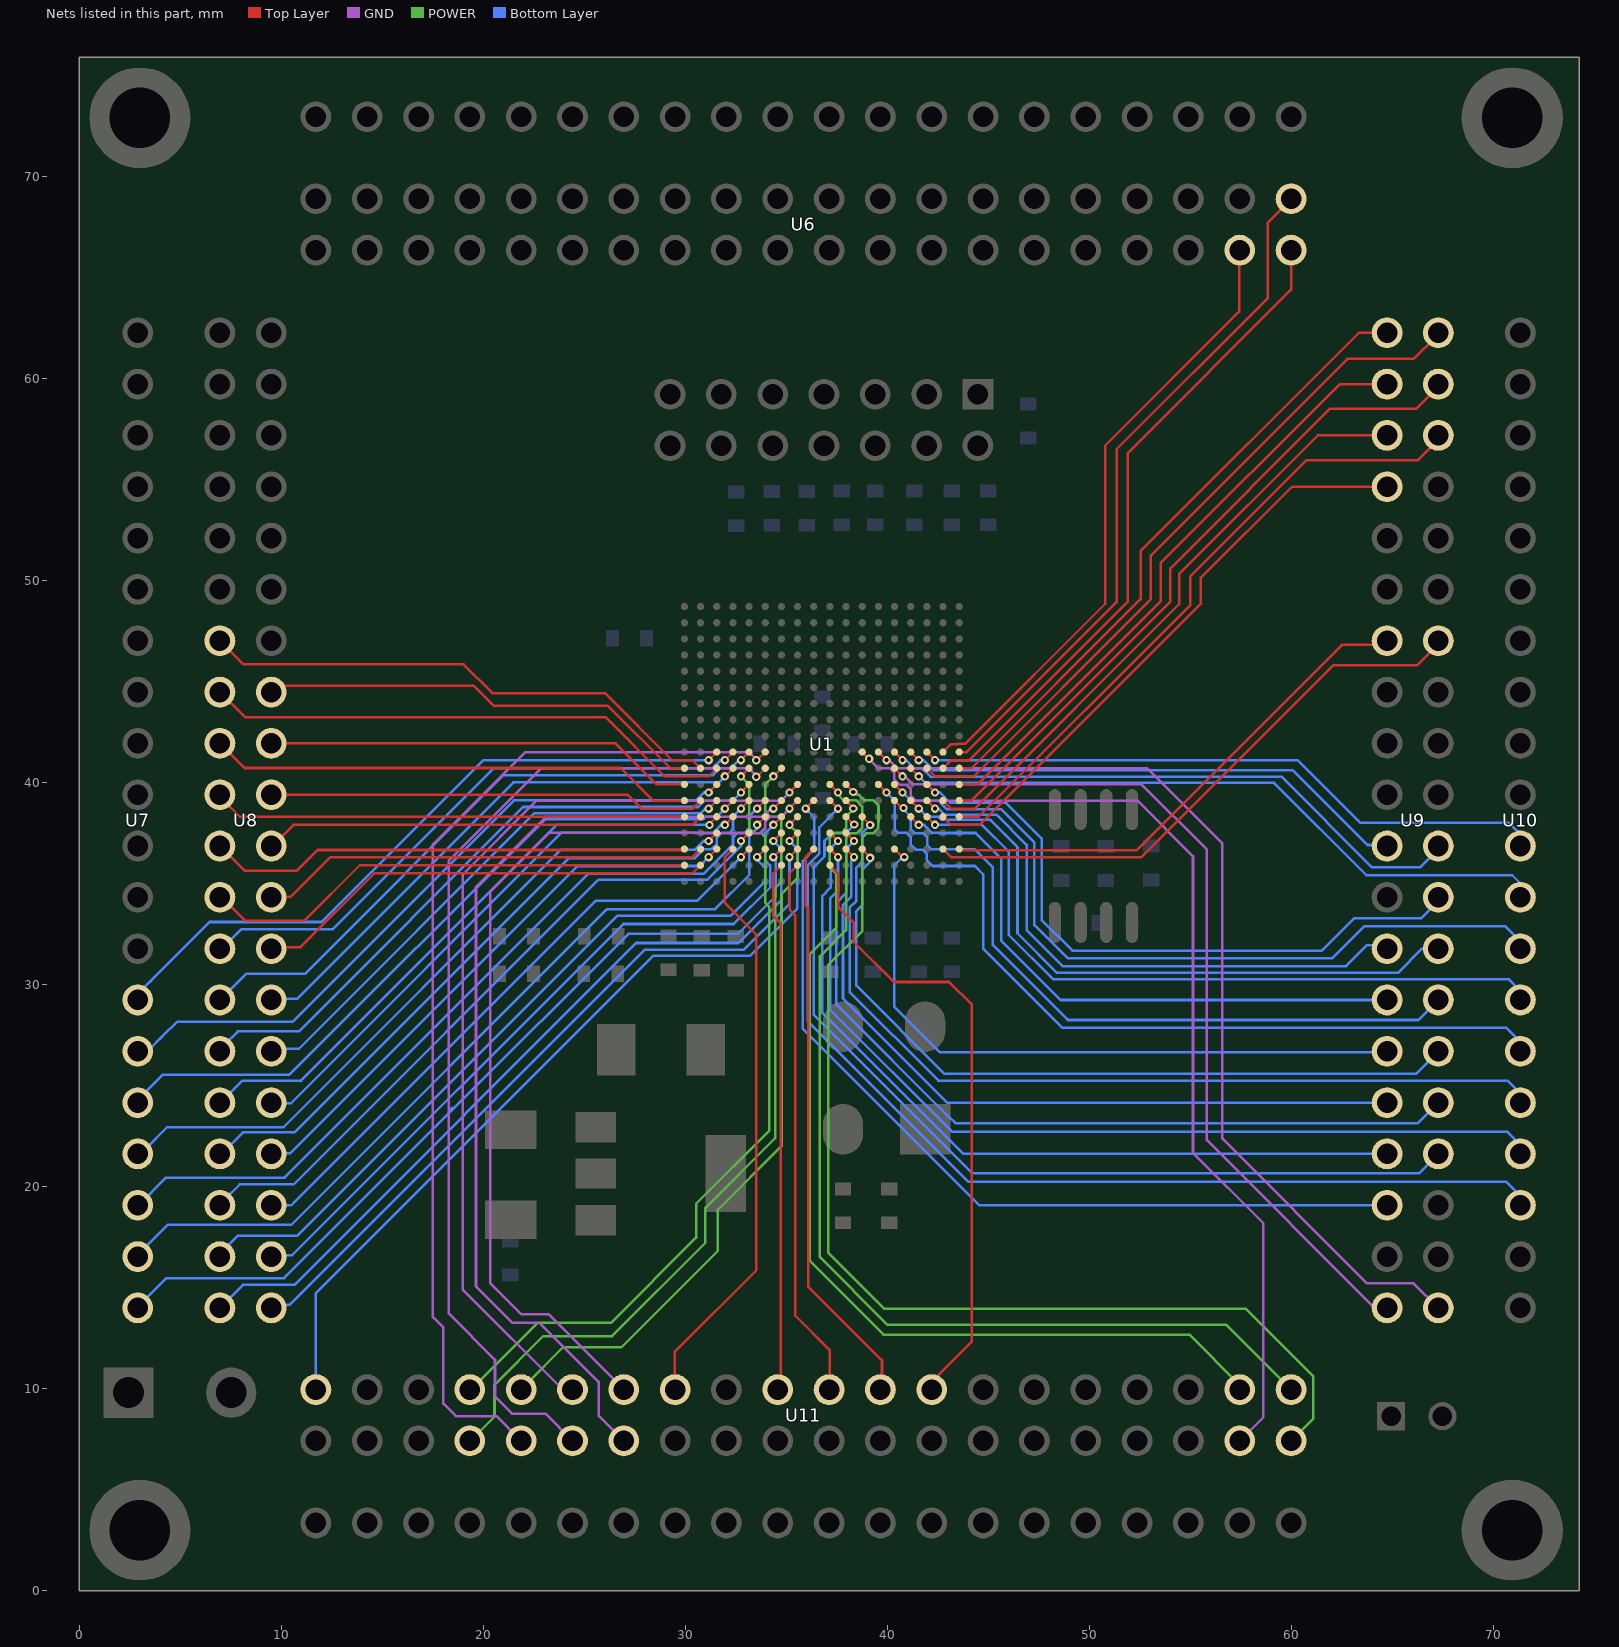
[diagram p0: the nets of this part, all layers, seen from the top]
# Altium PCB MISC103828.PcbDoc (part 3 of 4)
Units mm, origin at the board's own origin, x right, y up, seen from the top; angles counter-clockwise.
Board outline 74.24 x 75.89 mm, 4 copper layers (Top Layer, GND, POWER, Bottom Layer); 49 components, 246 nets, 670 pads, 283 vias.

## Via types
v1: diameter 0.406, hole 0.203, Top Layer to Bottom Layer, 221 vias
v2: diameter 0.61, hole 0.305, Top Layer to Bottom Layer, 43 vias
v3: diameter 0.508, hole 0.254, Top Layer to Bottom Layer, 16 vias
v4: diameter 0.432, hole 0.229, Top Layer to Bottom Layer, 3 vias

## Nets (pads, with @x,y where several pads share a name; then routed paths per layer and width w, separated by ;. In a path a pad name is that pad's centre, name@x,y a point inside that pad or via, vN(x,y) a via of type N, cw(c..) or ccw(c..) an arc to the next point about the centre after c; other vN are vias at no path point) (continued)
F_K3: U1.K3 U7.14 | length 34.1
  Top Layer w0.127: v1(31.147,41.103) U1.K3@31.547,41.503
  Bottom Layer w0.127: U7.14@2.845,29.286 2.845,29.489 3.556,30.201 ; 3.505,30.15 3.556,30.201 ; 22.993,41.103 23.139,41.103 ; v1(31.147,41.103) 23.139,41.103 ; 3.556,30.201 6.452,33.096 11.989,33.096 19.996,41.103 23.139,41.103
F_K4: U1.K4 U8.25 | length 29.1
  Top Layer w0.127: v1(31.947,41.103) U1.K4@32.347,41.503
  Bottom Layer w0.127: U8.25@7.239,31.953 8.014,32.728 12.535,32.728 20.517,40.71 31.337,40.71 31.725,41.097 v1@31.928,41.097 ; v1@31.935,41.09 v1(31.947,41.103)
F_K5: U1.K5 U8.27 | length 30.8
  Top Layer w0.127: v1(32.747,41.103) U1.K5@33.147,41.503
  Bottom Layer w0.127: U8.27@7.29,29.566 8.255,30.531 11.176,30.531 21.006,40.361 31.369,40.361 31.718,40.71 32.251,40.71 32.645,41.103 v1(32.747,41.103)
F_K6: U1.K6 U11.9 | length 51.3
  Top Layer w0.127: v1(33.503,41.097) 33.503,41.123 33.528,41.123 33.547,41.103 U1.K6@33.947,41.503
  GND w0.127: U11.9@21.869,7.417 20.65,8.636 18.644,8.636 18.021,9.258 18.021,13.018 17.501,13.538 17.501,36.932 22.073,41.504 33.147,41.504 33.528,41.123 33.503,41.123 v1(33.503,41.097)
F_K12: U1.K12 U11.37 | length 49.8
  Top Layer w0.127: U1.K12@38.747,41.503 39.091,41.16 v1(39.091,41.173)
  GND w0.127: v1(39.091,41.173) 39.091,41.16 39.554,40.697 40.11,40.697 40.341,40.466 40.341,40.153 40.597,39.897 40.91,39.897 41.141,39.666 41.141,39.353 41.397,39.097 52.368,39.097 55.118,36.347 55.118,21.666 58.598,18.186 58.598,8.585 U11.37@57.429,7.417
F_K13: U1.K13 U9.40 | length 47.7
  Top Layer w0.127: U1.K13@39.547,41.503 v1(39.947,41.103)
  GND w0.127: v1(39.947,41.103) 40.063,41.103 40.457,40.71 52.839,40.71 56.566,36.982 56.566,22.377 63.729,15.215 66.04,15.215 U9.40@67.259,13.995
F_K14: U1.K14 U9.22 | length 29.7
  Top Layer w0.127: U1.K14@40.347,41.503 v1(40.747,41.103)
  Bottom Layer w0.127: v1(40.747,41.103) 40.913,41.103 41.32,40.697 41.71,40.697 42.123,40.284 59.487,40.284 63.957,35.814 66.37,35.814 U9.22@67.335,36.779
F_K15: U1.K15 U9.21 | length 25.3
  Top Layer w0.127: U1.K15@41.147,41.503 v1(41.547,41.103)
  Bottom Layer w0.127: v1(41.547,41.103) 41.777,41.103 42.266,40.615 60.046,40.615 63.754,36.906 U9.21@64.567,36.906
F_K16: U1.K16 U10.11 | length 31.8
  Top Layer w0.127: U1.K16@41.947,41.503 v1(42.347,41.103)
  Bottom Layer w0.127: v1(42.347,41.103) 60.293,41.103 63.398,37.998 70.764,37.998 U10.11@71.857,36.906
F_K17: U1.K17 U6.37 | length 31.1
  Top Layer w0.127: U1.K17@42.747,41.503 43.143,41.899 43.485,41.899 43.485,41.907 43.838,41.907 50.775,48.844 50.775,56.667 57.404,63.297 57.404,66.015 U6.37@57.353,66.065
F_K18: U1.K18 U6.40 | length 34.5
  Top Layer w0.127: U1.K18@43.547,41.503 43.916,41.503 51.333,48.92 51.333,56.49 58.826,63.983 58.826,67.71 59.249,68.132 ; 59.293,68.177 59.249,68.132 ; U6.40@59.969,68.936 59.969,68.853 59.249,68.132
F_L1: U1.L1 U8.16 | length 22.3
  Top Layer w0.127: U8.16@9.5,44.475 9.804,44.78 19.533,44.78 19.837,44.475 19.875,44.437 20.523,43.79 26.162,43.79 29.248,40.703 U1.L1@29.947,40.703
F_L2: U1.L2 U8.13 | length 26.4
  Top Layer w0.127: U8.13@6.96,47.015 8.128,45.847 19.025,45.847 20.447,44.425 26.01,44.425 29.335,41.099 30.352,41.099 U1.L2@30.747,40.703
F_L3: U1.L3 U8.15 | length 26.5
  Top Layer w0.127: U8.15@6.96,44.475 8.204,43.231 26.035,43.231 28.958,40.307 30.111,40.307 30.114,40.31 30.581,40.31 30.583,40.307 31.152,40.307 U1.L3@31.547,40.703
F_L4: U1.L4 U8.28 | length 27.4
  Top Layer w0.127: v1(31.947,40.303) U1.L4@32.347,40.703
  Bottom Layer w0.127: U8.28@9.677,29.286 10.77,29.286 21.488,40.005 31.649,40.005 v1(31.947,40.303)
F_L5: U1.L5 U11.8 | length 39.6
  Top Layer w0.127: v1(32.747,40.303) U1.L5@33.147,40.703
  POWER w0.127: U11.8@19.66,10.236 22.682,13.259 26.314,13.259 30.531,17.475 30.531,19.152 34.138,22.758 34.138,33.858 33.954,34.042 33.954,37.266 33.967,37.28 33.75,37.497 33.397,37.497 33.154,37.74 33.154,39.897 v1(32.747,40.303)
F_L6: U1.L6 U11.11 | length 50.3
  Top Layer w0.127: v1(33.503,40.284) 33.494,40.284 33.494,40.252 33.496,40.252 U1.L6@33.947,40.703
  GND w0.127: U11.11@24.409,7.417 23.063,8.763 21.412,8.763 20.574,9.601 20.574,11.43 18.288,13.716 18.288,36.144 22.841,40.697 33.154,40.697 33.547,40.303 33.496,40.252 33.494,40.252 33.494,40.284 v1(33.503,40.284)
F_L7: U1.L7 U11.7 | length 42.7
  Top Layer w0.127: v1(34.347,40.303) U1.L7@34.747,40.703
  POWER w0.127: U11.7@19.228,7.29 20.549,8.611 20.549,10.185 22.962,12.598 26.365,12.598 30.988,17.221 30.988,18.948 34.442,22.403 34.442,34.239 34.442,34.315 34.442,34.773 34.747,35.077 34.747,38.125 34.563,38.31 34.184,38.31 33.941,38.553 33.941,38.583 33.941,39.897 v1(34.347,40.303)
F_L14: U1.L14 U9.39 | length 43.9
  Top Layer w0.127: U1.L14@40.347,40.703 v1(40.747,40.303)
  GND w0.127: v1(40.747,40.303) 40.863,40.303 41.263,39.903 52.578,39.903 55.804,36.678 55.804,22.301 64.11,13.995 U9.39@64.719,13.995
F_L15: U1.L15 U10.12 | length 33.3
  Top Layer w0.127: U1.L15@41.147,40.703 v1(41.547,40.303)
  Bottom Layer w0.127: v1(41.547,40.303) 41.871,39.98 59.131,39.98 63.703,35.408 70.917,35.408 U10.12@71.857,34.468
F_L16: U1.L16 U9.2 | length 35.7
  Top Layer w0.127: U1.L16@41.947,40.703 42.343,40.307 44.27,40.307 53.035,49.073 53.035,51.232 62.763,60.96 64.465,60.96 66.04,60.96 U9.2@67.208,62.128
F_L17: U1.L17 U6.39 | length 33.2
  Top Layer w0.127: U1.L17@42.747,40.703 43.129,41.085 43.37,41.085 43.383,41.099 43.711,41.099 43.725,41.085 44.032,41.085 51.892,48.946 51.892,56.312 59.969,64.389 59.969,66.142 U6.39@60.046,66.218
F_L18: U1.L18 U9.1 | length 31.5
  Top Layer w0.127: U1.L18@43.547,40.703 44.158,40.703 52.527,49.073 52.527,51.46 63.322,62.255 U9.1@64.719,62.255
F_M1: U1.M1 U8.18 | length 21.3
  Top Layer w0.127: U8.18@9.5,41.935 26.543,41.935 28.575,39.903 U1.M1@29.947,39.903
F_M3: U1.M3 U7.15 | length 34.1
  Top Layer w0.127: v1(31.147,39.503) U1.M3@31.547,39.903
  Bottom Layer w0.127: U7.15@3.099,26.822 3.505,26.822 4.102,27.419 ; 3.988,27.305 4.102,27.419 ; 24.098,39.11 24.155,39.11 ; v1(31.147,39.503) 30.918,39.503 30.525,39.11 24.155,39.11 ; 4.102,27.419 4.851,28.169 10.566,28.169 21.508,39.11 24.155,39.11
F_M5: U1.M5 U8.29 | length 31.3
  Top Layer w0.127: v1(32.747,39.503) U1.M5@33.147,39.903
  Bottom Layer w0.127: U8.29@7.188,27.026 7.849,27.686 10.871,27.686 21.971,38.786 30.632,38.786 30.944,39.097 32.341,39.097 v1(32.747,39.503)
F_M8: U1.M8 U11.12 | length 46.4
  Top Layer w0.127: v1(35.147,39.503) U1.M8@35.547,39.903
  GND w0.127: U11.12@24.409,9.957 23.927,9.957 18.974,14.91 18.974,35.433 22.638,39.097 34.741,39.097 v1(35.147,39.503)
F_M10: U1.M10 U11.40 | length 51.4
  Top Layer w0.127: U1.M10@37.147,39.903 v1(37.547,39.503)
  POWER w0.127: v1@37.541,39.395 37.808,39.129 38.441,39.129 38.748,38.822 38.748,37.757 38.633,37.643 ; 38.638,37.638 38.498,37.497 38.184,37.497 37.954,37.266 37.954,32.696 36.652,31.394 36.652,16.51 40.005,13.157 56.769,13.157 U11.40@59.969,9.957
F_M11: U1.M11 U11.39 | length 55.7
  Top Layer w0.127: U1.M11@37.947,39.903 v1@38.341,39.51
  POWER w0.127: v1(38.303,39.522) 38.303,39.472 38.316,39.472 38.347,39.503 38.379,39.471 38.379,39.446 38.443,39.383 38.597,39.383 38.87,39.11 39.298,39.11 39.554,38.854 39.554,38.028 39.535,38.009 39.535,37.734 39.298,37.497 38.984,37.497 38.748,37.26 38.748,35.82 38.754,35.814 38.754,32.658 37.059,30.963 37.059,16.739 39.853,13.945 57.734,13.945 61.062,10.617 61.062,8.509 U11.39@59.969,7.417
F_M13: U1.M13 U10.15 | length 41.1
  Top Layer w0.127: U1.M13@39.547,39.903 v1(39.947,39.503)
  Bottom Layer w0.127: v1(39.947,39.503) 40.361,39.09 40.361,38.873 40.354,38.866 40.354,37.675 40.519,37.51 40.91,37.51 40.917,37.516 40.919,37.516 41.141,37.294 41.141,36.94 41.14,36.939 41.402,36.677 41.73,36.677 41.948,36.459 41.948,36.146 42.229,35.865 44.323,35.865 44.729,35.458 44.729,31.775 48.641,27.864 70.612,27.864 U10.15@71.78,26.695
F_M14: U1.M14 U10.13 | length 38.2
  Top Layer w0.127: U1.M14@40.347,39.903 v1(40.747,39.503)
  Bottom Layer w0.127: v1(40.747,39.503) 41.154,39.097 42.51,39.097 42.796,38.811 42.799,38.811 42.945,38.665 45.637,38.665 47.269,37.033 47.269,32.944 48.92,31.293 62.001,31.293 63.602,32.893 70.561,32.893 U10.13@71.501,31.953
F_M16: U1.M16 U9.24 | length 32
  Top Layer w0.127: U1.M16@41.947,39.903 v1(42.347,39.503)
  Bottom Layer w0.127: v1(42.347,39.503) 42.589,39.503 43.104,38.989 45.872,38.989 47.625,37.236 47.625,33.198 49.149,31.674 61.493,31.674 63.094,33.274 66.396,33.274 U9.24@67.208,34.087
F_M18: U1.M18 U9.3 | length 30.7
  Top Layer w0.127: U1.M18@43.547,39.903 44.45,39.903 53.53,48.984 ; 53.518,48.997 53.518,50.851 62.382,59.715 U9.3@64.719,59.715 ; U9.3@64.719,59.639 U9.3@64.922,59.639
F_N1: U1.N1 U8.17 | length 24.2
  Top Layer w0.127: U8.17@6.96,41.935 8.179,40.716 26.797,40.716 28.397,39.116 ; 28.397,39.103 U1.N1@29.947,39.103
F_N2: U1.N2 U8.20 | length 21.7
  Top Layer w0.127: U8.20@9.5,39.395 27.127,39.395 27.815,38.708 30.352,38.708 U1.N2@30.747,39.103
F_N3: U1.N3 U8.30 | length 27
  Top Layer w0.127: v1(31.147,38.703) U1.N3@31.547,39.103
  Bottom Layer w0.127: U8.30@9.601,26.822 10.871,26.822 22.53,38.481 30.759,38.481 30.982,38.703 v1(31.147,38.703)
F_N4: U1.N4 U7.16 | length 35.6
  Top Layer w0.127: v1(31.947,38.703) U1.N4@32.347,39.103
  Bottom Layer w0.127: U7.16@2.921,24.206 U7.16@3.277,24.206 ; U7.16@3.099,24.511 4.115,25.527 10.389,25.527 23.038,38.176 30.863,38.176 30.984,38.297 31.541,38.297 v1(31.947,38.703)
F_N5: U1.N5 U8.33 | length 33.5
  Top Layer w0.127: v1(32.747,38.703) U1.N5@33.147,39.103
  Bottom Layer w0.127: U8.33@7.341,21.92 8.103,22.682 10.643,22.682 24.206,36.246 30.455,36.246 30.906,36.697 31.298,36.697 31.554,36.953 31.554,37.269 31.795,37.51 32.176,37.51 32.36,37.694 32.36,37.734 32.354,37.74 32.354,38.066 32.36,38.072 32.36,38.316 v1(32.747,38.703)
F_N6: U1.N6 U7.18 | length 39.9
  Top Layer w0.127: v1(33.547,38.703) U1.N6@33.947,39.103
  Bottom Layer w0.127: U7.18@2.921,19.075 4.293,20.447 5.969,20.447 10.16,20.447 25.197,35.484 30.912,35.484 32.361,36.933 32.354,36.94 32.354,37.281 32.583,37.511 32.584,37.51 32.91,37.51 33.154,37.753 33.154,38.31 v1(33.547,38.703)
F_N7: U1.N7 U11.13 | length 48.1
  Top Layer w0.127: v1(34.347,38.703) U1.N7@34.747,39.103
  GND w0.127: U11.13@26.949,7.417 25.705,8.661 25.705,10.338 22.784,13.259 21.438,13.259 19.634,15.062 19.634,34.823 23.121,38.31 33.838,38.31 34.231,38.703 v1(34.347,38.703)
F_N8: U1.N8 U11.14 | length 45.4
  Top Layer w0.127: v1(35.147,38.703) U1.N8@35.547,39.103
  GND w0.127: U11.14@26.949,9.957 23.216,13.691 21.869,13.691 20.345,15.215 20.345,34.595 23.254,37.503 30.491,37.503 30.497,37.497 33.698,37.497 33.941,37.74 33.941,38.054 34.184,38.297 34.741,38.297 v1(35.147,38.703)
F_N9: U1.N9 U9.35 | length 44.4
  Top Layer w0.127: v1(35.947,38.703) U1.N9@36.347,39.103
  Bottom Layer w0.127: v1(35.947,38.703) 36.373,38.278 36.373,36.678 35.795,36.1 35.795,27.832 44.552,19.075 U9.35@64.719,19.075
F_N10: U1.N10 U10.18 | length 51.2
  Top Layer w0.127: U1.N10@37.147,39.103 v1(37.547,38.703)
  Bottom Layer w0.127: v1(37.547,38.703) 36.627,37.783 36.627,36.474 36.049,35.897 36.049,28.187 43.993,20.244 70.612,20.244 U10.18@71.78,19.075
F_N11: U1.N11 U11.38 | length 48.4
  Top Layer w0.127: U1.N11@37.947,39.103 v1@38.322,38.729 ; v1(38.303,38.71) v1@38.322,38.729 ; v1@38.322,38.729 38.329,38.735 38.329,38.722 v1@38.322,38.729
  POWER w0.127: 37.948,38.303 37.948,37.747 37.71,37.51 37.397,37.51 37.135,37.248 37.135,35.789 37.465,35.458 37.465,32.817 36.144,31.496 36.144,16.332 39.802,12.675 54.94,12.675 57.429,10.185 U11.38@57.429,9.957 ; 37.954,38.303 37.954,38.309 v1@38.354,38.71
F_N14: U1.N14 U9.28 | length 34.8
  Top Layer w0.127: U1.N14@40.347,39.103 40.747,38.703 40.767,38.723 40.767,38.735 v1(40.792,38.735)
  Bottom Layer w0.127: v1(40.792,38.735) 40.767,38.735 40.767,38.723 40.747,38.703 41.148,38.303 41.148,37.694 41.344,37.497 41.751,37.497 41.974,37.274 41.974,36.908 41.966,36.901 42.164,36.703 44.298,36.703 45.212,35.789 45.212,31.953 48.92,28.245 66.269,28.245 U9.28@67.259,29.235
F_N15: U1.N15 U9.26 | length 32.6
  Top Layer w0.127: U1.N15@41.147,39.103 v1(41.547,38.703)
  Bottom Layer w0.127: v1(41.547,38.703) 41.948,38.303 42.504,38.303 42.65,38.157 45.078,38.157 46.431,36.805 46.431,32.537 48.387,30.582 65.253,30.582 66.446,31.775 U9.26@67.259,31.775
F_N16: U1.N16 U9.25 | length 29.4
  Top Layer w0.127: U1.N16@41.947,39.103 v1(42.347,38.703)
  Bottom Layer w0.127: v1(42.347,38.703) 42.526,38.703 42.818,38.411 45.383,38.411 46.888,36.906 46.888,32.69 48.666,30.912 62.687,30.912 63.729,31.953 U9.25@65.024,31.953
F_N17: U1.N17 U9.5 | length 30.7
  Top Layer w0.127: U1.N17@42.747,39.103 43.143,38.708 44.321,38.708 54.432,48.819 54.432,50.317 61.29,57.175 U9.5@64.719,57.175
F_N18: U1.N18 U9.4 | length 33.2
  Top Layer w0.127: U1.N18@43.547,39.103 44.158,39.103 54,48.946 54,50.597 61.9,58.496 66.167,58.496 U9.4@67.259,59.588
F_P1: U1.P1 U8.19 | length 23.1
  Top Layer w0.127: U8.19@7.137,39.116 7.95,38.303 U1.P1@29.947,38.303
F_P2: U1.P2 U8.22 | length 21.6
  Top Layer w0.127: U8.22@9.754,37.059 10.594,37.899 15.215,37.899 ; 15.116,37.899 15.215,37.899 ; U1.P2@30.747,38.303 30.343,37.899 15.215,37.899
F_P3: U1.P3 U8.31 | length 30.3
  Top Layer w0.127: v1(31.191,37.897) 31.154,37.897 31.147,37.903 U1.P3@31.547,38.303
  Bottom Layer w0.127: U8.31@7.112,24.282 8.077,25.248 10.973,25.248 23.629,37.903 31.147,37.903 31.154,37.897 v1(31.191,37.897)
F_P4: U1.P4 U8.32 | length 28.8
  Top Layer w0.127: v1(31.947,37.903) U1.P4@32.347,38.303
  Bottom Layer w0.127: U8.32@9.525,24.13 10.49,24.13 23.876,37.516 30.912,37.516 30.924,37.503 31.356,37.503 31.757,37.903 v1(31.947,37.903) 31.915,37.871 v1@31.953,37.871
F_P6: U1.P6 U7.19 | length 41.3
  Top Layer w0.127: v1(33.547,37.903) U1.P6@33.947,38.303
  Bottom Layer w0.127: U7.19@2.946,16.688 4.369,18.11 10.49,18.11 26.111,33.731 31.471,33.731 33.147,35.408 33.147,37.313 33.547,37.713 v1(33.547,37.903) ; U7.19@3.277,16.612 U7.19@3.277,16.688
F_P7: U1.P7 U8.38 | length 36.2
  Top Layer w0.127: v1(34.347,37.903) U1.P7@34.747,38.303
  Bottom Layer w0.127: U8.38@9.423,16.612 10.541,16.612 26.924,32.995 32.385,32.995 34.195,34.805 34.195,35.899 33.954,36.14 33.954,37.51 v1(34.347,37.903)
F_P8: U1.P8 U11.10 | length 35.6
  Top Layer w0.127: v1(35.147,37.903) U1.P8@35.547,38.303
  POWER w0.127: U11.10@22.174,10.287 23.927,12.04 26.822,12.04 31.598,16.815 31.598,18.847 34.754,22.003 34.754,34.474 ; 34.747,34.468 34.754,34.474 ; v1(35.147,37.903) 35.554,37.497 35.554,35.274 34.754,34.474
F_P11: U1.P11 U9.34 | length 45.8
  Top Layer w0.127: U1.P11@37.947,38.303 38.347,37.903 38.354,37.91 v1(38.354,37.922)
  Bottom Layer w0.127: v1(38.354,37.922) 38.354,37.91 37.941,37.497 37.269,37.497 36.881,37.109 36.881,36.347 36.357,35.824 36.357,28.489 44.196,20.65 66.294,20.65 U9.34@67.259,21.615
F_P12: U1.P12 U10.16 | length 45.3
  Top Layer w0.127: U1.P12@38.747,38.303 39.129,37.922 39.141,37.922 v1(39.141,37.897)
  Bottom Layer w0.127: v1(39.141,37.897) 39.141,37.922 39.129,37.922 39.147,37.903 38.741,37.497 38.741,36.14 38.722,36.122 38.722,36.083 38.736,36.069 38.456,35.789 38.456,34.138 38.125,33.807 38.125,29.642 42.52,25.248 70.688,25.248 U10.16@71.78,24.155
F_P15: U1.P15 U9.27 | length 29.7
  Top Layer w0.127: U1.P15@41.147,38.303 v1(41.547,37.903)
  Bottom Layer w0.127: v1(41.547,37.903) 41.594,37.903 v1@41.601,37.897 ; v1@41.58,37.897 v1@41.601,37.897 ; 42.197,37.497 41.954,37.74 41.954,37.752 41.808,37.897 v1@41.601,37.897 ; 42.198,37.497 42.204,37.503 42.53,37.503 42.536,37.497 42.986,37.497 42.988,37.5 44.364,37.5 45.618,36.246 45.618,32.182 48.565,29.235 U9.27@64.719,29.235
F_P16: U1.P16 U10.14 | length 36
  Top Layer w0.127: U1.P16@41.947,38.303 v1(42.347,37.903)
  Bottom Layer w0.127: v1(42.347,37.903) 44.672,37.903 45.999,36.576 45.999,32.461 48.209,30.251 70.764,30.251 U10.14@71.78,29.235
F_P17: U1.P17 U9.7 | length 29.6
  Top Layer w0.127: U1.P17@42.747,38.303 43.151,37.899 44.554,37.899 55.512,48.857 ; 55.499,48.87 55.499,50.114 60.02,54.635 61.747,54.635 U9.7@64.541,54.635
F_P18: U1.P18 U9.6 | length 32.1
  Top Layer w0.127: U1.P18@43.547,38.303 44.501,38.303 54.991,48.793 54.991,50.216 60.731,55.956 66.243,55.956 U9.6@67.107,56.82
F_R3: U1.R3 U7.17 | length 34.7
  Top Layer w0.127: v1(31.147,37.103) U1.R3@31.547,37.503
  Bottom Layer w0.127: U7.17@3.302,21.895 4.343,22.936 10.109,22.936 23.851,36.678 30.472,36.678 30.898,37.103 v1(31.147,37.103)
F_R5: U1.R5 U8.35 | length 33.9
  Top Layer w0.127: v1(32.747,37.103) U1.R5@33.147,37.503
  Bottom Layer w0.127: U8.35@6.934,19.202 U8.35@7.112,19.38 ; U8.35@7.163,19.329 7.95,20.117 10.617,20.117 25.679,35.179 31.064,35.179 32.747,36.862 v1(32.747,37.103)
F_R7: U1.R7 U8.39 | length 39.6
  Top Layer w0.127: v1(34.347,37.103) U1.R7@34.747,37.503
  Bottom Layer w0.127: U8.39@7.061,14.148 U8.39@7.137,14.224 ; U8.39@7.163,14.199 8.103,15.138 10.643,15.138 27.559,32.055 32.614,32.055 34.747,34.188 34.747,36.704 v1(34.347,37.103)
F_R8: U1.R8 U11.2 | length 40.2
  Top Layer w0.127: v1(35.147,37.103) U1.R8@35.547,37.503
  Bottom Layer w0.127: U11.2@11.76,10.363 11.709,10.414 11.709,14.732 28.397,31.42 33.198,31.42 35.541,33.763 35.541,36.71 v1(35.147,37.103)
F_R10: U1.R10 U9.33 | length 40.3
  Top Layer w0.127: U1.R10@37.147,37.503 v1(37.547,37.103)
  Bottom Layer w0.127: v1(37.547,37.103) 37.135,36.691 37.135,36.017 37.186,35.966 37.186,34.798 36.779,34.392 36.779,28.6 43.764,21.615 U9.33@64.719,21.615
F_R11: U1.R11 U9.32 | length 41.7
  Top Layer w0.127: U1.R11@37.947,37.503 v1(38.347,37.103)
  Bottom Layer w0.127: v1(38.347,37.103) 37.948,36.704 37.948,34.519 37.465,34.036 37.465,29.007 42.989,23.482 ; 43.002,23.495 43.358,23.139 66.243,23.139 U9.32@67.259,24.155
F_T1: U1.T1 U8.21 | length 23.7
  Top Layer w0.127: U8.21@7.163,36.652 8.179,35.636 10.77,35.636 11.792,36.659 15.011,36.659 ; 14.917,36.659 15.011,36.659 ; U1.T1@29.947,36.703 29.903,36.659 15.011,36.659
F_T2: U1.T2 U8.24 | length 22.3
  Top Layer w0.127: U8.24@9.398,34.341 10.465,34.341 12.432,36.308 30.352,36.308 U1.T2@30.747,36.703
F_T3: U1.T3 U8.34 | length 28.4
  Top Layer w0.127: v1(31.147,36.303) U1.T3@31.547,36.703
  Bottom Layer w0.127: U8.34@9.423,21.641 10.439,21.641 24.663,35.865 26.543,35.865 ; 26.467,35.865 26.543,35.865 ; v1(31.147,36.303) 30.709,35.865 26.543,35.865
F_T4: U1.T4 U11.16 | length 28.8
  Top Layer w0.127: U11.16@29.464,10.363 29.464,11.811 33.503,15.85 33.503,32.487 31.952,34.038 31.952,36.308 U1.T4@32.347,36.703
F_T5: U1.T5 U8.36 | length 30.9
  Top Layer w0.127: v1(32.747,36.303) U1.T5@33.147,36.703
  Bottom Layer w0.127: U8.36@9.5,19.075 10.49,19.075 10.643,19.228 10.693,19.279 25.552,34.138 30.582,34.138 v1(32.747,36.303)
F_T6: U1.T6 U8.37 | length 36.5
  Top Layer w0.127: v1(33.547,36.303) U1.T6@33.947,36.703
  Bottom Layer w0.127: U8.37@6.985,16.713 7.849,17.577 10.795,17.577 26.619,33.401 32.233,33.401 33.941,35.11 33.941,35.782 33.547,36.176 v1(33.547,36.303)
F_T7: U1.T7 U7.20 | length 42.8
  Top Layer w0.127: v1(34.347,36.303) U1.T7@34.747,36.703
  Bottom Layer w0.127: U7.20@2.743,13.894 4.318,15.469 10.135,15.469 18.453,23.787 27.178,32.512 32.588,32.512 34.468,34.392 34.468,35.89 34.468,35.966 34.468,36.195 v1@34.366,36.297 ; 18.402,23.838 18.453,23.889 ; v1@34.347,36.297 v1(34.347,36.303)
F_T8: U1.T8 U8.40 | length 36.7
  Top Layer w0.127: v1(35.147,36.303) U1.T8@35.547,36.703
  Bottom Layer w0.127: U8.40@9.55,14.148 10.414,14.148 19.469,23.203 27.991,31.725 32.893,31.725 35.147,33.979 v1(35.147,36.303)
F_T9: U1.T9 U11.24 | length 28.2
  Top Layer w0.127: U1.T9@36.347,36.703 35.947,36.303 35.947,33.903 36.068,33.782 36.068,15.062 39.726,11.405 U11.24@39.726,10.185
F_T10: U1.T10 U10.17 | length 45.9
  Top Layer w0.127: U1.T10@37.147,36.703 v1(37.547,36.303)
  Bottom Layer w0.127: v1(37.547,36.303) 37.547,34.652 37.16,34.265 37.16,28.753 43.205,22.708 70.688,22.708 U10.17@71.78,21.615
F_T11: U1.T11 U9.31 | length 36.9
  Top Layer w0.127: U1.T11@37.947,36.703 v1(38.347,36.303)
  Bottom Layer w0.127: v1@38.379,36.322 38.379,36.297 38.202,36.119 38.202,34.341 37.795,33.934 37.795,29.312 42.951,24.155 U9.31@64.719,24.155
F_T12: U1.T12 U9.30 | length 38.5
  Top Layer w0.127: U1.T12@38.747,36.703 39.179,36.272 v1(39.141,36.271)
  Bottom Layer w0.127: v1(39.141,36.271) 39.179,36.271 39.147,36.303 39.147,36.113 39.167,36.093 38.754,35.68 38.754,33.928 38.456,33.63 38.456,29.947 42.824,25.578 66.142,25.578 U9.30@67.259,26.695
F_T14: U1.T14 U9.29 | length 33.6
  Top Layer w0.127: U1.T14@40.347,36.703 40.747,36.303 v1@40.767,36.323 ; v1@40.767,36.322 40.792,36.297 40.818,36.322 40.875,36.322 40.875,36.303 v1(40.826,36.303)
  Bottom Layer w0.127: v1@40.767,36.322 40.792,36.297 40.818,36.322 40.875,36.322 40.875,36.303 v1(40.826,36.303) ; v1@40.767,36.323 40.322,35.879 40.322,28.918 42.596,26.645 U9.29@64.44,26.645
F_T17: U1.T17 U9.14 | length 29.2
  Top Layer w0.127: U1.T17@42.747,36.703 43.154,36.297 43.381,36.297 43.383,36.299 43.711,36.299 43.714,36.297 52.553,36.297 62.052,45.796 66.192,45.796 U9.14@67.361,46.965
F_T18: U1.T18 U9.13 | length 25.5
  Top Layer w0.127: U1.T18@43.547,36.703 43.611,36.639 52.311,36.639 62.484,46.812 U9.13@64.821,46.812
F_U1: U1.U1 U8.23 | length 24.3
  Top Layer w0.127: U8.23@7.188,34.188 8.23,33.147 11.125,33.147 13.882,35.903 U1.U1@29.947,35.903
F_U2: U1.U2 U8.26 | length 22.8
  Top Layer w0.127: U8.26@9.677,31.852 10.947,31.852 14.603,35.508 16.916,35.508 ; 16.864,35.508 16.916,35.508 ; U1.U2@30.747,35.903 30.352,35.508 16.916,35.508
F_U7: U1.U7 U11.20 | length 25.9
  Top Layer w0.127: U11.20@34.696,10.389 34.722,10.414 34.722,12.675 ; 34.722,12.624 34.722,12.675 ; U1.U7@34.747,35.903 34.352,35.508 34.352,33.39 34.722,33.02 34.722,12.675
F_U8: U1.U8 U11.22 | length 27
  Top Layer w0.127: 35.433,14.097 35.433,14.173 ; U1.U8@35.547,35.903 35.152,35.508 35.152,33.708 35.433,33.426 35.433,14.173 ; U11.22@37.135,9.957 37.135,11.913 35.433,13.614 35.433,14.173
F_U10: U1.U10 U11.26 | length 30.8
  Top Layer w0.127: U1.U10@37.147,35.903 37.551,35.499 37.551,33.848 38.329,33.071 38.329,32.106 40.31,30.124 43.053,30.124 44.171,29.007 44.171,12.344 U11.26@42.266,10.439